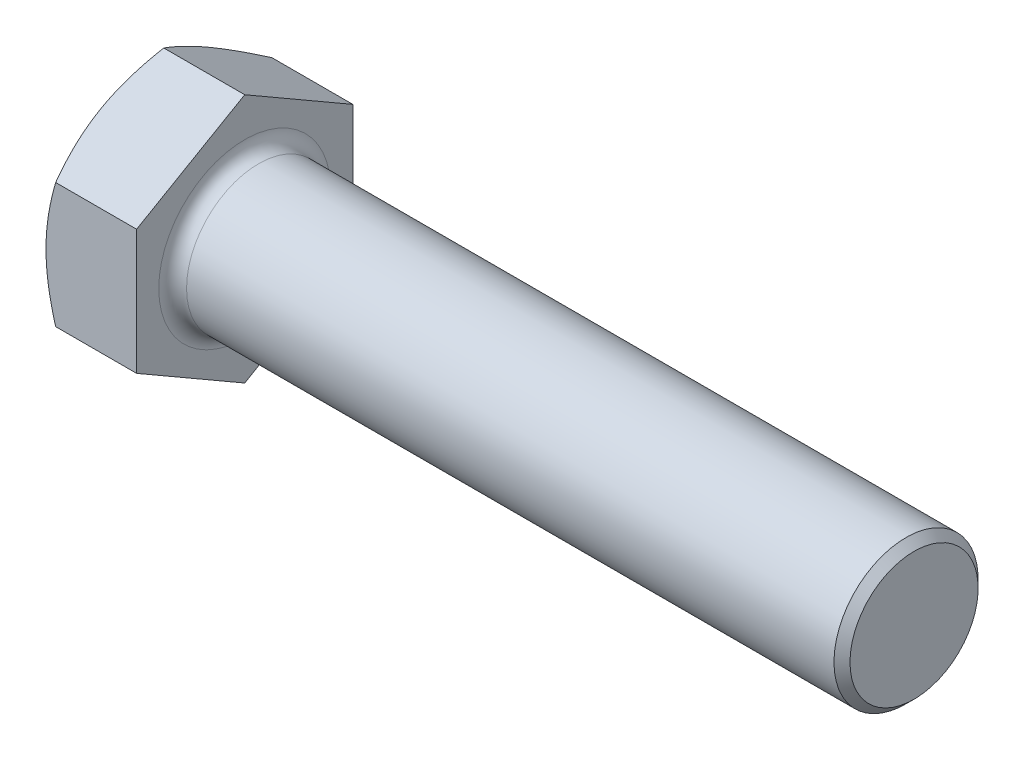
from build123d import *

# Parameters (mm, degrees)
BOSS_EXTRUDE1_DEPTH = 8.8
SKETCH4_R           = 22.78
SKETCH4_R_2         = 10.5
CUT_EXTRUDE1_DEPTH  = 1.1
CUT_EXTRUDE1_DRAFT  = -60
CHAMFER2_SIZE       = 0.777777778


with BuildPart() as part:
    # Sketch3 → Boss-Extrude1 (new body)
    with BuildSketch(Plane(origin=(0, 0, 0), x_dir=(0, 0, -1), z_dir=(1, 0, 0))):
        Polygon((10.5, 6.062177826), (0, 12.124355653), (-10.5, 6.062177826), (-10.5, -6.062177826), (0, -12.124355653), (10.5, -6.062177826), align=None)
    extrude(amount=BOSS_EXTRUDE1_DEPTH)


with BuildPart() as cut_extrude1_tool:
    # Sketch4 → Cut-Extrude1 (with draft: the straight prism first)
    with BuildSketch(Plane.ZY):
        Circle(SKETCH4_R)
        Circle(SKETCH4_R_2, mode=Mode.SUBTRACT)
    extrude(amount=-CUT_EXTRUDE1_DEPTH)
    # Cut-Extrude1: the draft: its side faces are tilted about the plane it starts from
    cut_extrude1_sides = [cut_extrude1_tool.faces().sort_by_distance(p)[0] for p in [
        (0.55, 0, -22.78),
        (0.55, 0, -10.5),
    ]]
    draft(cut_extrude1_sides, Plane.ZY, CUT_EXTRUDE1_DRAFT)


with BuildPart() as part_1:
    add(part.part)

    # Cut-Extrude1: cut by cut_extrude1_tool
    add(cut_extrude1_tool.part, mode=Mode.SUBTRACT)

    # Sketch5 → Revolve1 (revolve)
    with BuildSketch(Plane.XY, mode=Mode.PRIVATE) as revolve1_sk:
        with BuildLine():
            Line((10.15, 7), (73.8, 7))
            Line((73.8, 7), (73.8, 0))
            Line((73.8, 0), (8.8, 0))
            Line((8.8, 0), (8.8, 8.35))
            ThreePointArc((8.8, 8.35), (9.195405845, 7.395405845), (10.15, 7))
        make_face()
    revolve(revolve1_sk.sketch.rotate(Axis((8.8, 0, 0), (1, 0, 0)), 90), axis=Axis((8.8, 0, 0), (1, 0, 0)))

    # Chamfer2
    chamfer2_edges = [part_1.edges().sort_by_distance(p)[0] for p in [
        (73.8, 0, -7),
    ]]
    chamfer(chamfer2_edges, length=CHAMFER2_SIZE)


solid = part_1.part
